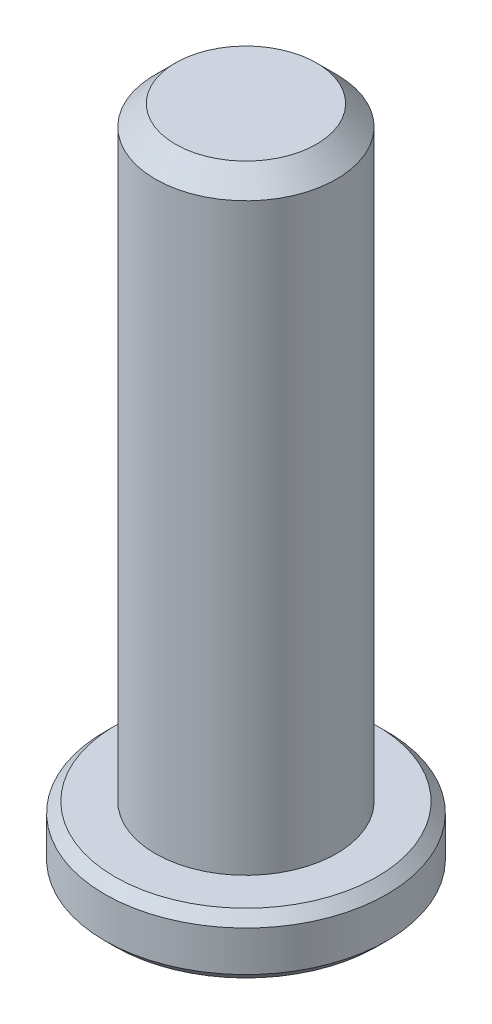
from build123d import *

# Parameters (mm, degrees)
SKETCH1_R           = 7
BOSS_EXTRUDE1_DEPTH = 3
SKETCH2_R           = 4.5
BOSS_EXTRUDE2_DEPTH = 30
CHAMFER1_SIZE       = 1
CHAMFER2_SIZE       = 0.5


with BuildPart() as part:
    # Sketch1 → Boss-Extrude1 (new body)
    with BuildSketch(Plane(origin=(0, 0, 0), x_dir=(1, 0, 0), z_dir=(0, 1, 0))):
        with Locations(Location((0, 0, 0), (0, 0, 270))):
            Circle(SKETCH1_R)
    extrude(amount=BOSS_EXTRUDE1_DEPTH)

    # Sketch2 → Boss-Extrude2 (add)
    with BuildSketch(Plane(origin=(0, 3, 0), x_dir=(1, 0, 0), z_dir=(0, 1, 0))):
        with Locations(Location((0, 0, 0), (0, 0, 270))):
            Circle(SKETCH2_R)
    extrude(amount=BOSS_EXTRUDE2_DEPTH)

    # Chamfer1
    chamfer1_edges = [part.edges().sort_by_distance(p)[0] for p in [
        (0, 33, -4.5),
    ]]
    chamfer(chamfer1_edges, length=CHAMFER1_SIZE)

    # Chamfer2
    chamfer2_edges = [part.edges().sort_by_distance(p)[0] for p in [
        (0, 0, -7),
        (0, 3, -7),
    ]]
    chamfer(chamfer2_edges, length=CHAMFER2_SIZE)


solid = part.part
